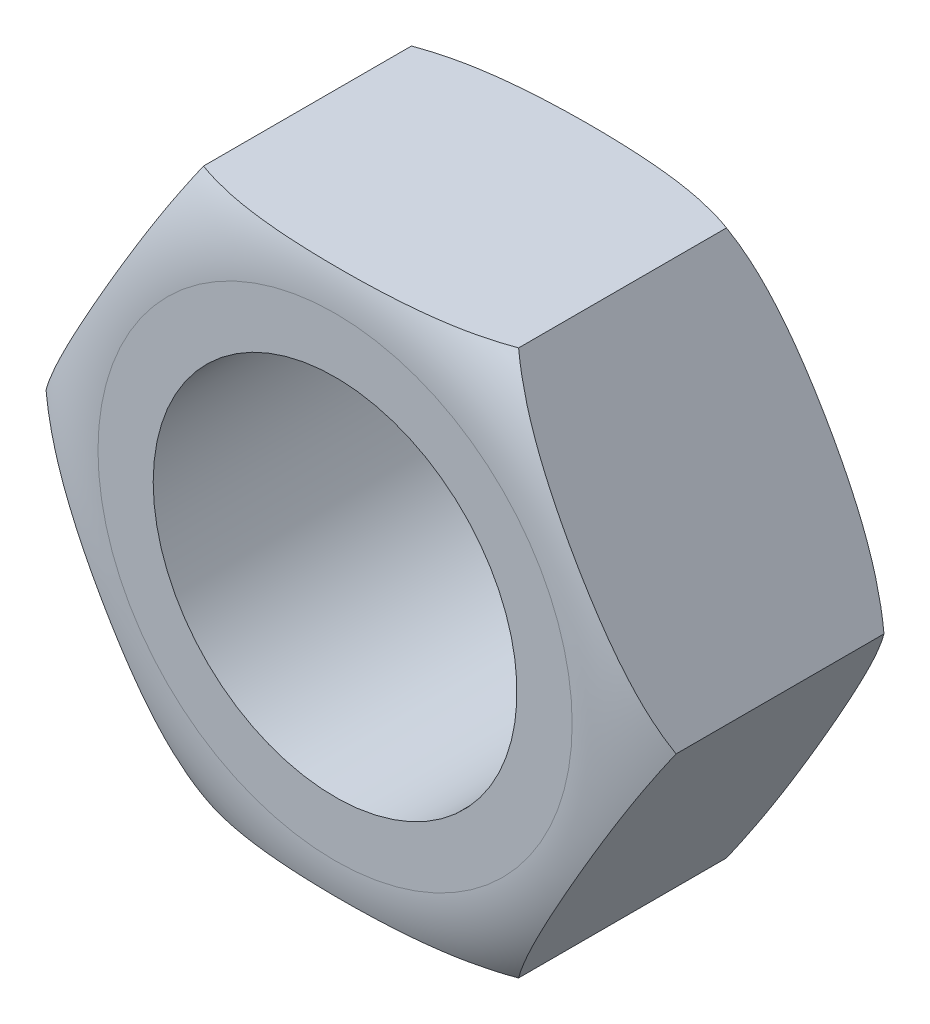
SolidWorks part; units mm, degrees
ref_plane "Front" through (0, 0, 0) normal (0, 0, 1) x (1, 0, 0)
ref_plane "Top" through (0, 0, 0) normal (0, 1, 0) x (1, 0, 0)
ref_plane "Right" through (0, 0, 0) normal (1, 0, 0) x (0, 0, -1)
sketch "Sketch1" plane through (0, 0, 0) normal (0, 0, 1) x (1, 0, 0)
  line L1 (12.1244, 0) -> (6.0622, 10.5)
  line L2 (6.0622, 10.5) -> (-6.0622, 10.5)
  line L3 (-6.0622, 10.5) -> (-12.1244, 0)
  line L4 (-12.1244, 0) -> (-6.0622, -10.5)
  line L5 (-6.0622, -10.5) -> (6.0622, -10.5)
  line L6 (6.0622, -10.5) -> (12.1244, 0)
  circle A0 centre (0, 0) radius 10.5 construction
  dimension "D1" = 21
extrude "Boss-Extrude1" add sketch "Sketch1" along normal blind 10
sketch "Sketch2" plane through (0, 0, 0) normal (0, 1, 0) x (1, 0, 0)
  line L0 (-12.1244, 0) -> (-12.1244, -1)
  line L1 (-12.1244, -10) -> (-12.1244, 0) construction
  line L2 (-12.1244, 0) -> (-9.1244, 0)
  line L3 (0, 0) -> (0, -6.8929) construction
  line L4 (-15.0287, -5) -> (16.4628, -5) construction
  line L7 (-12.1244, -10) -> (-12.1244, -9)
  line L8 (-12.1244, -10) -> (-9.1244, -10)
  arc A0 (-12.1244, -1) -> (-9.1244, 0) centre (-9.1244, -5) cw
  arc A1 (-12.1244, -9) -> (-9.1244, -10) centre (-9.1244, -5) ccw
  dimension "D3" = 5
  dimension "D1" = 1
  dimension "D2" = 3
revolve "Cut-Revolve1" cut sketch "Sketch2" angle 360 about L3
sketch "Sketch3" plane through (0, 0, 0) normal (0, 0, -1) x (-1, 0, 0)
  circle A0 centre (0, 0) radius 7
  dimension "D1" = 14
extrude "Cut-Extrude1" cut sketch "Sketch3" against normal blind 10
